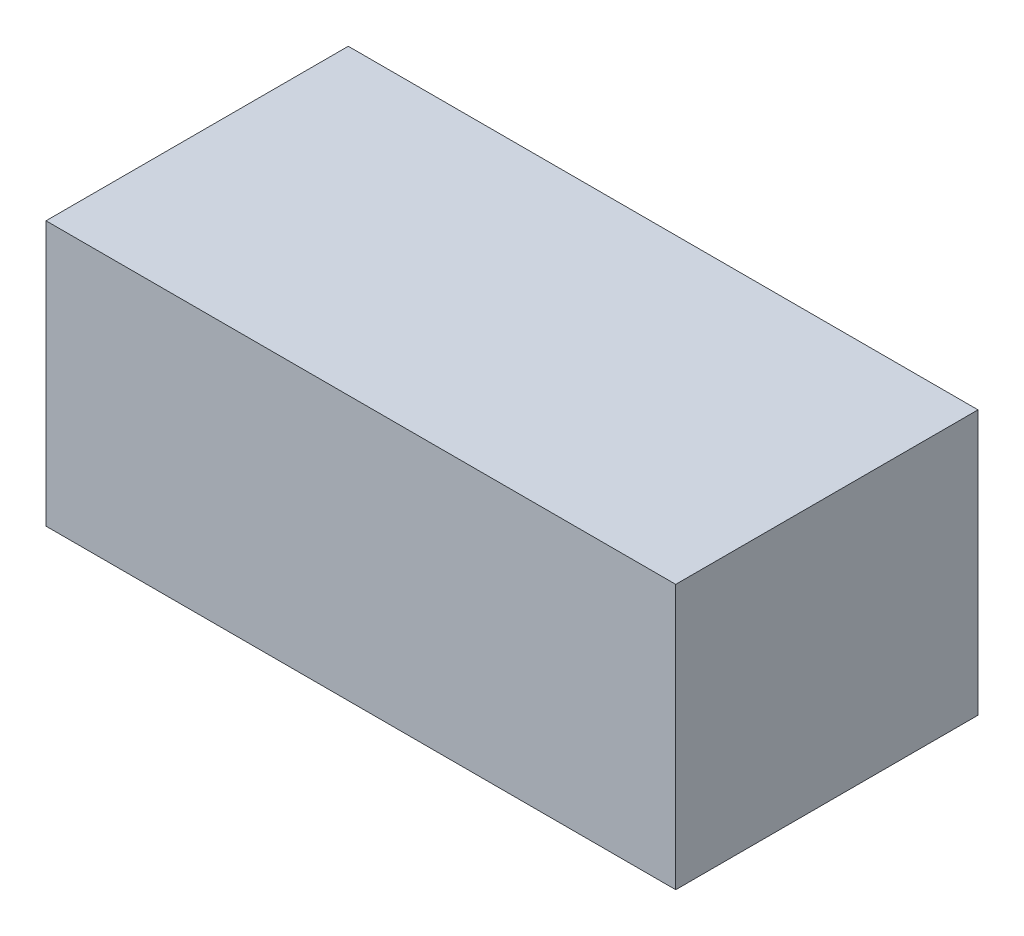
from build123d import *

# Parameters (mm, degrees)
SKETCH_1_W      = 25
SKETCH_1_H      = 10.5
EXTRUDE_1_DEPTH = 6


with BuildPart() as part:
    # 草图1 → 凸台-拉伸1 (new, symmetric)
    with BuildSketch(Plane.XY):
        Rectangle(SKETCH_1_W, SKETCH_1_H)
    extrude(amount=EXTRUDE_1_DEPTH, both=True)


solid = part.part
